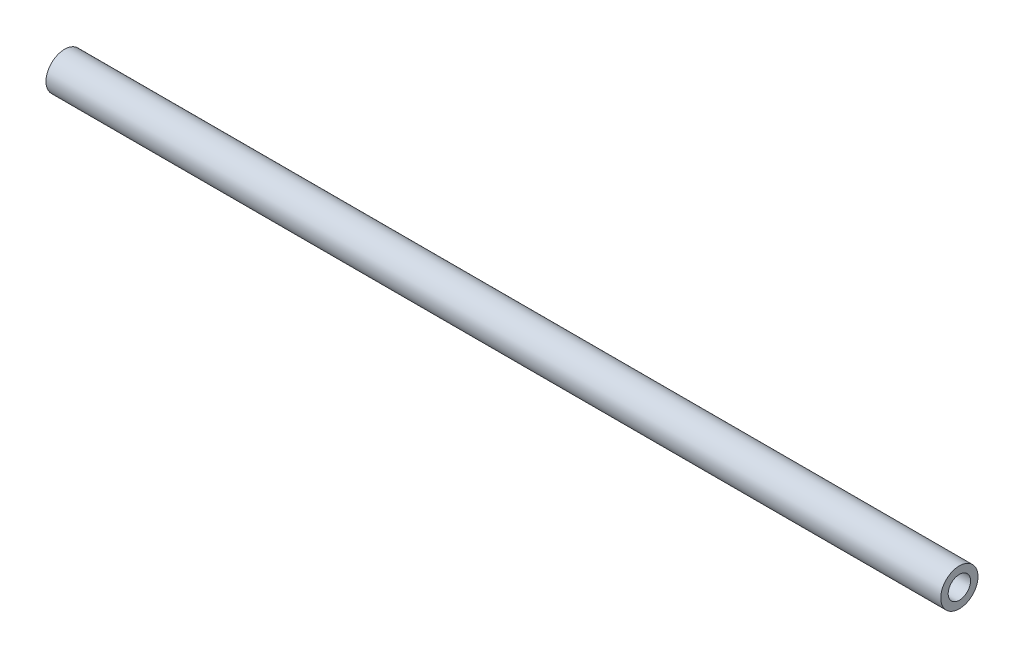
from build123d import *

# Parameters (mm, degrees)
SKETCH_1_R      = 2.5
SKETCH_1_R_2    = 1.5
EXTRUDE_1_DEPTH = 120


with BuildPart() as part:
    # 草图1 → 凸台-拉伸1 (new body)
    with BuildSketch(Plane(origin=(0, 0, 0), x_dir=(0, 0, -1), z_dir=(1, 0, 0))):
        Circle(SKETCH_1_R)
        Circle(SKETCH_1_R_2, mode=Mode.SUBTRACT)
    extrude(amount=EXTRUDE_1_DEPTH)


solid = part.part
